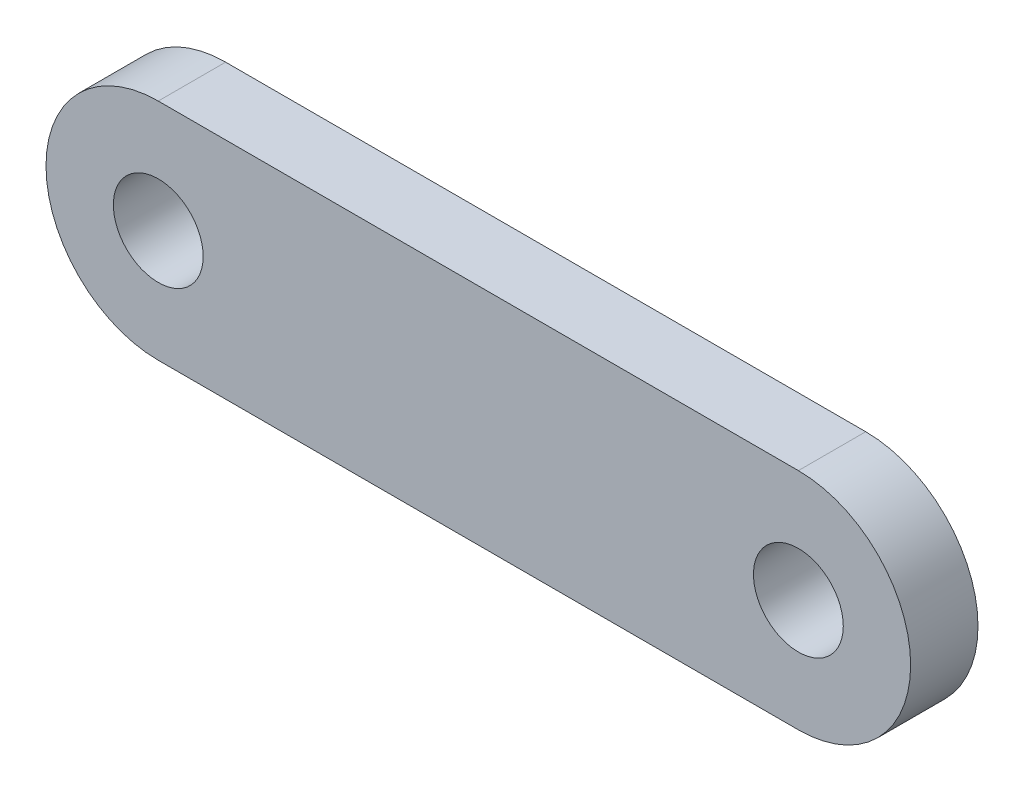
from build123d import *

# Parameters (mm, degrees)
BOSS_EXTRUDE1_DEPTH = 6
SKETCH2_R           = 4
CUT_EXTRUDE1_DEPTH  = 95


with BuildPart() as part:
    # Sketch1 → Boss-Extrude1 (new body)
    with BuildSketch(Plane.XY):
        with BuildLine():
            Line((0, 10), (57.02, 10))
            ThreePointArc((57.02, 10), (67.02, 0), (57.02, -10))
            Line((57.02, -10), (0, -10))
            ThreePointArc((0, -10), (-10, 0), (0, 10))
        make_face()
    extrude(amount=BOSS_EXTRUDE1_DEPTH)

    # Sketch2 → Cut-Extrude1 (cut)
    with BuildSketch(Plane.XY.offset(6)):
        Circle(SKETCH2_R)
        with Locations((57.02, 0)):
            Circle(SKETCH2_R)
    extrude(amount=-CUT_EXTRUDE1_DEPTH, mode=Mode.SUBTRACT)


solid = part.part
